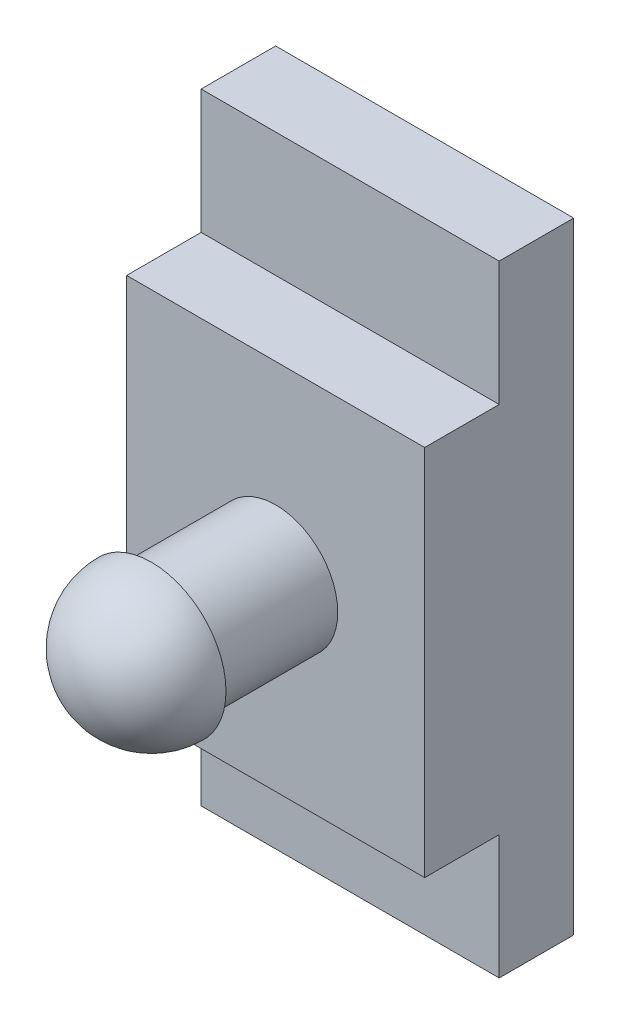
SolidWorks part; units mm, degrees
ref_plane "Front Plane" through (0, 0, 0) normal (0, 0, 1) x (1, 0, 0)
ref_plane "Top Plane" through (0, 0, 0) normal (0, 1, 0) x (1, 0, 0)
ref_plane "Right Plane" through (0, 0, 0) normal (1, 0, 0) x (0, 0, -1)
sketch "Sketch1" plane through (0, 0, 0) normal (0, 0, 1) x (1, 0, 0)
  line L1 (-6, 12.5) -> (6, 12.5)
  line L2 (-6, 12.5) -> (-6, -12.5)
  line L3 (-6, -12.5) -> (6, -12.5)
  line L4 (6, 12.5) -> (6, -12.5)
  line L5 (-6, 12.5) -> (6, -12.5) construction
  line L6 (-6, -12.5) -> (6, 12.5) construction
  point P0 (0, 0)
  dimension "D1" = 12
  dimension "D2" = 25
extrude "Boss-Extrude1" add sketch "Sketch1" along normal blind 3
sketch "Sketch2" plane through (0, 0, 3) normal (0, 0, 1) x (1, 0, 0)
  line L0 (6, -12.5) -> (6, 12.5) construction
  line L1 (-6, -7.5) -> (6, -7.5)
  line L2 (-6, -7.5) -> (-6, 7.5)
  line L3 (-6, 7.5) -> (6, 7.5)
  line L4 (6, -7.5) -> (6, 7.5)
  line L5 (-6, -7.5) -> (6, 7.5) construction
  line L6 (-6, 7.5) -> (6, -7.5) construction
  point P0 (0, 0)
  dimension "D1" = 15
extrude "Boss-Extrude2" add sketch "Sketch2" along normal blind 3
sketch "Sketch3" plane through (0, 0, 6) normal (0, 0, 1) x (1, 0, 0)
  circle A0 centre (0, 0) radius 2.5
  dimension "D1" = 5
extrude "Boss-Extrude3" add sketch "Sketch3" along normal blind 5
sketch "Sketch4" plane through (0, 0, 0) normal (0, 1, 0) x (1, 0, 0)
  line L0 (0, -11) -> (3, -11)
  line L1 (-2.5, -11) -> (2.5, -11) construction
  line L2 (0, -11) -> (0, -14)
  arc A0 (3, -11) -> (0, -14) centre (0, -11) cw
  dimension "D1" = 3
revolve "Revolve1" add sketch "Sketch4" angle 360 about L2
scale "Scale1" bodies to scale 104 scale about origin uniform scaling yes scale factor 2.5
